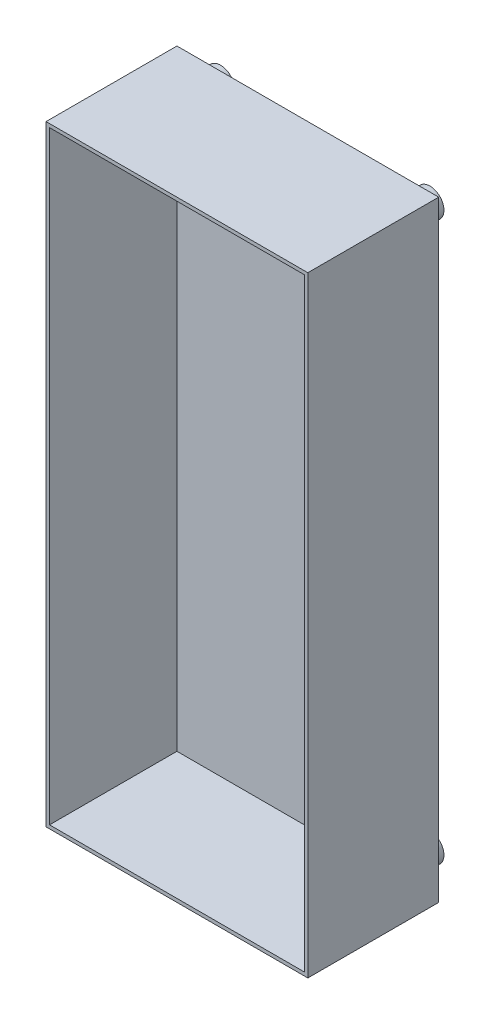
SolidWorks part; units mm, degrees
ref_plane "Front Plane" through (0, 0, 0) normal (0, 0, 1) x (1, 0, 0)
ref_plane "Top Plane" through (0, 0, 0) normal (0, 1, 0) x (1, 0, 0)
ref_plane "Right Plane" through (0, 0, 0) normal (1, 0, 0) x (0, 0, -1)
sketch "Sketch1" plane through (0, 0, 0) normal (0, 0, 1) x (1, 0, 0)
  line L1 (75, 175) -> (-75, 175)
  line L2 (75, 175) -> (75, -175)
  line L3 (75, -175) -> (-75, -175)
  line L4 (-75, 175) -> (-75, -175)
  line L5 (75, 175) -> (-75, -175) construction
  line L6 (75, -175) -> (-75, 175) construction
  point P0 (0, 0)
  dimension "D1" = 150
  dimension "D2" = 350
extrude "Boss-Extrude1" add sketch "Sketch1" along normal blind 75
shell "Shell1" thickness 2
sketch "Sketch2" plane through (0, 0, 0) normal (0, 0, -1) x (-1, 0, 0)
  line L0 (0, 0) -> (0, 43.4021) construction
  line L1 (-62.9734, 154.85) -> (-57.0266, 154.85)
  line L2 (-57.0266, 154.85) -> (-54.0533, 160)
  line L3 (-54.0533, 160) -> (-57.0266, 165.15)
  line L4 (-57.0266, 165.15) -> (-62.9734, 165.15)
  line L5 (-62.9734, 165.15) -> (-65.9467, 160)
  line L6 (-65.9467, 160) -> (-62.9734, 154.85)
  line L7 (60, -160) -> (-60, -160) construction
  line L8 (60, -160) -> (60, 160) construction
  line L9 (60, 160) -> (-60, 160) construction
  line L10 (-60, -160) -> (-60, 160) construction
  line L11 (60, -160) -> (-60, 160) construction
  line L12 (60, 160) -> (-60, -160) construction
  line L13 (0, 0) -> (19.161, 0) construction
  line L14 (-65.9467, -160) -> (-62.9734, -154.85)
  line L15 (-62.9734, -165.15) -> (-65.9467, -160)
  line L16 (-57.0266, -165.15) -> (-62.9734, -165.15)
  line L17 (-54.0533, -160) -> (-57.0266, -165.15)
  line L18 (-57.0266, -154.85) -> (-54.0533, -160)
  line L19 (-62.9734, -154.85) -> (-57.0266, -154.85)
  line L20 (62.9734, -165.15) -> (65.9467, -160)
  line L21 (57.0266, -165.15) -> (62.9734, -165.15)
  line L22 (54.0533, -160) -> (57.0266, -165.15)
  line L23 (57.0266, -154.85) -> (54.0533, -160)
  line L24 (62.9734, -154.85) -> (57.0266, -154.85)
  line L25 (65.9467, -160) -> (62.9734, -154.85)
  line L26 (65.9467, 160) -> (62.9734, 154.85)
  line L27 (62.9734, 165.15) -> (65.9467, 160)
  line L28 (57.0266, 165.15) -> (62.9734, 165.15)
  line L29 (54.0533, 160) -> (57.0266, 165.15)
  line L30 (57.0266, 154.85) -> (54.0533, 160)
  line L31 (62.9734, 154.85) -> (57.0266, 154.85)
  circle A0 centre (-60, 160) radius 8
  circle A1 centre (-60, 160) radius 5.15 construction
  circle A2 centre (-60, -160) radius 8
  circle A3 centre (60, -160) radius 8
  circle A4 centre (60, 160) radius 8
  point P2 (0, 0)
  dimension "D1" = 16
  dimension "D2" = 10.3
  dimension "D3" = 120
  dimension "D4" = 320
extrude "Boss-Extrude2" add sketch "Sketch2" along normal blind 10
